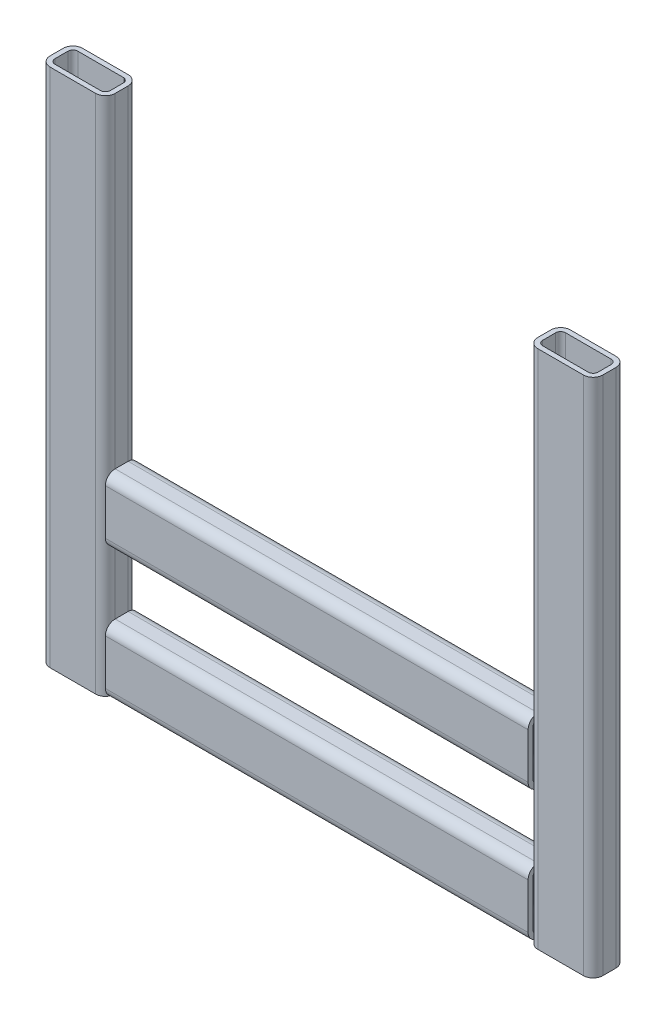
from build123d import *

# Parameters (mm, degrees)
F_40_X_20_X_3_1_DEPTH      = 300
F_40_X_20_X_3_1_DEPTH_BACK = 20
F_40_X_20_X_3_1_2_DEPTH    = 320
F_40_X_20_X_3_1_3_DEPTH    = 302
F_40_X_20_X_3_1_4_DEPTH    = 302


with BuildPart() as part:
    # Sketch1 → 矩形管 40 X 20 X 3(1) (new, two sides: drawn at the far end of the back side and taken through both)
    with BuildSketch(Plane(origin=(0, 0, 0), x_dir=(0, 0, -1), z_dir=(0, 1, 0)).offset(-F_40_X_20_X_3_1_DEPTH_BACK)):
        with BuildLine():
            Line((-4, -20), (4, -20))
            ThreePointArc((4, -20), (8.242640687, -18.242640687), (10, -14))
            Line((10, -14), (10, 14))
            ThreePointArc((10, 14), (8.242640687, 18.242640687), (4, 20))
            Line((4, 20), (-4, 20))
            ThreePointArc((-4, 20), (-8.242640687, 18.242640687), (-10, 14))
            Line((-10, 14), (-10, -14))
            ThreePointArc((-10, -14), (-8.242640687, -18.242640687), (-4, -20))
        make_face()
        with BuildLine():
            Line((-4, -17), (4, -17))
            ThreePointArc((4, -17), (6.121320344, -16.121320344), (7, -14))
            Line((7, -14), (7, 14))
            ThreePointArc((7, 14), (6.121320344, 16.121320344), (4, 17))
            Line((4, 17), (-4, 17))
            ThreePointArc((-4, 17), (-6.121320344, 16.121320344), (-7, 14))
            Line((-7, 14), (-7, -14))
            ThreePointArc((-7, -14), (-6.121320344, -16.121320344), (-4, -17))
        make_face(mode=Mode.SUBTRACT)
    extrude(amount=F_40_X_20_X_3_1_DEPTH + F_40_X_20_X_3_1_DEPTH_BACK)


with BuildPart() as body_2:
    # Sketch1 on segment 2 (carried to segment 2) → 40 X 20 X 3_1 2 (new body)
    with BuildSketch(Plane(origin=(300, -20, 0), x_dir=(0, 0, -1), z_dir=(0, 1, 0))):
        with BuildLine():
            Line((-4, -20), (4, -20))
            ThreePointArc((4, -20), (8.242640687, -18.242640687), (10, -14))
            Line((10, -14), (10, 14))
            ThreePointArc((10, 14), (8.242640687, 18.242640687), (4, 20))
            Line((4, 20), (-4, 20))
            ThreePointArc((-4, 20), (-8.242640687, 18.242640687), (-10, 14))
            Line((-10, 14), (-10, -14))
            ThreePointArc((-10, -14), (-8.242640687, -18.242640687), (-4, -20))
        make_face()
        with BuildLine():
            Line((-4, -17), (4, -17))
            ThreePointArc((4, -17), (6.121320344, -16.121320344), (7, -14))
            Line((7, -14), (7, 14))
            ThreePointArc((7, 14), (6.121320344, 16.121320344), (4, 17))
            Line((4, 17), (-4, 17))
            ThreePointArc((-4, 17), (-6.121320344, 16.121320344), (-7, 14))
            Line((-7, 14), (-7, -14))
            ThreePointArc((-7, -14), (-6.121320344, -16.121320344), (-4, -17))
        make_face(mode=Mode.SUBTRACT)
    extrude(amount=F_40_X_20_X_3_1_2_DEPTH)


with BuildPart() as body_3:
    # Sketch1 on segment 3 (carried to segment 3) → 40 X 20 X 3_1 3 (new body)
    with BuildSketch(Plane(origin=(-1, 0, 0), x_dir=(0, 0, -1), z_dir=(1, 0, 0))):
        with BuildLine():
            Line((-4, -20), (4, -20))
            ThreePointArc((4, -20), (8.242640687, -18.242640687), (10, -14))
            Line((10, -14), (10, 14))
            ThreePointArc((10, 14), (8.242640687, 18.242640687), (4, 20))
            Line((4, 20), (-4, 20))
            ThreePointArc((-4, 20), (-8.242640687, 18.242640687), (-10, 14))
            Line((-10, 14), (-10, -14))
            ThreePointArc((-10, -14), (-8.242640687, -18.242640687), (-4, -20))
        make_face()
        with BuildLine():
            Line((-4, -17), (4, -17))
            ThreePointArc((4, -17), (6.121320344, -16.121320344), (7, -14))
            Line((7, -14), (7, 14))
            ThreePointArc((7, 14), (6.121320344, 16.121320344), (4, 17))
            Line((4, 17), (-4, 17))
            ThreePointArc((-4, 17), (-6.121320344, 16.121320344), (-7, 14))
            Line((-7, 14), (-7, -14))
            ThreePointArc((-7, -14), (-6.121320344, -16.121320344), (-4, -17))
        make_face(mode=Mode.SUBTRACT)
    extrude(amount=F_40_X_20_X_3_1_3_DEPTH)

    # 40 X 20 X 3_1 3 end butt 1
    split(bisect_by=Plane.YZ.offset(20), keep=Keep.TOP)

    # 40 X 20 X 3_1 3 end butt 2
    split(bisect_by=Plane(origin=(280, 0, 0), x_dir=(0, -1, 0), z_dir=(-1, 0, 0)), keep=Keep.TOP)


with BuildPart() as body_4:
    # Sketch1 on segment 4 (carried to segment 4) → 40 X 20 X 3_1 4 (new body)
    with BuildSketch(Plane(origin=(-1, 80, 0), x_dir=(0, 0, -1), z_dir=(1, 0, 0))):
        with BuildLine():
            Line((-4, -20), (4, -20))
            ThreePointArc((4, -20), (8.242640687, -18.242640687), (10, -14))
            Line((10, -14), (10, 14))
            ThreePointArc((10, 14), (8.242640687, 18.242640687), (4, 20))
            Line((4, 20), (-4, 20))
            ThreePointArc((-4, 20), (-8.242640687, 18.242640687), (-10, 14))
            Line((-10, 14), (-10, -14))
            ThreePointArc((-10, -14), (-8.242640687, -18.242640687), (-4, -20))
        make_face()
        with BuildLine():
            Line((-4, -17), (4, -17))
            ThreePointArc((4, -17), (6.121320344, -16.121320344), (7, -14))
            Line((7, -14), (7, 14))
            ThreePointArc((7, 14), (6.121320344, 16.121320344), (4, 17))
            Line((4, 17), (-4, 17))
            ThreePointArc((-4, 17), (-6.121320344, 16.121320344), (-7, 14))
            Line((-7, 14), (-7, -14))
            ThreePointArc((-7, -14), (-6.121320344, -16.121320344), (-4, -17))
        make_face(mode=Mode.SUBTRACT)
    extrude(amount=F_40_X_20_X_3_1_4_DEPTH)

    # 40 X 20 X 3_1 4 end butt 1
    split(bisect_by=Plane(origin=(20, 80, 0), x_dir=(0, 1, 0), z_dir=(1, 0, 0)), keep=Keep.TOP)

    # 40 X 20 X 3_1 4 end butt 2
    split(bisect_by=Plane(origin=(280, 80, 0), x_dir=(0, -1, 0), z_dir=(-1, 0, 0)), keep=Keep.TOP)


solid = Compound([part.part, body_2.part, body_3.part, body_4.part])
